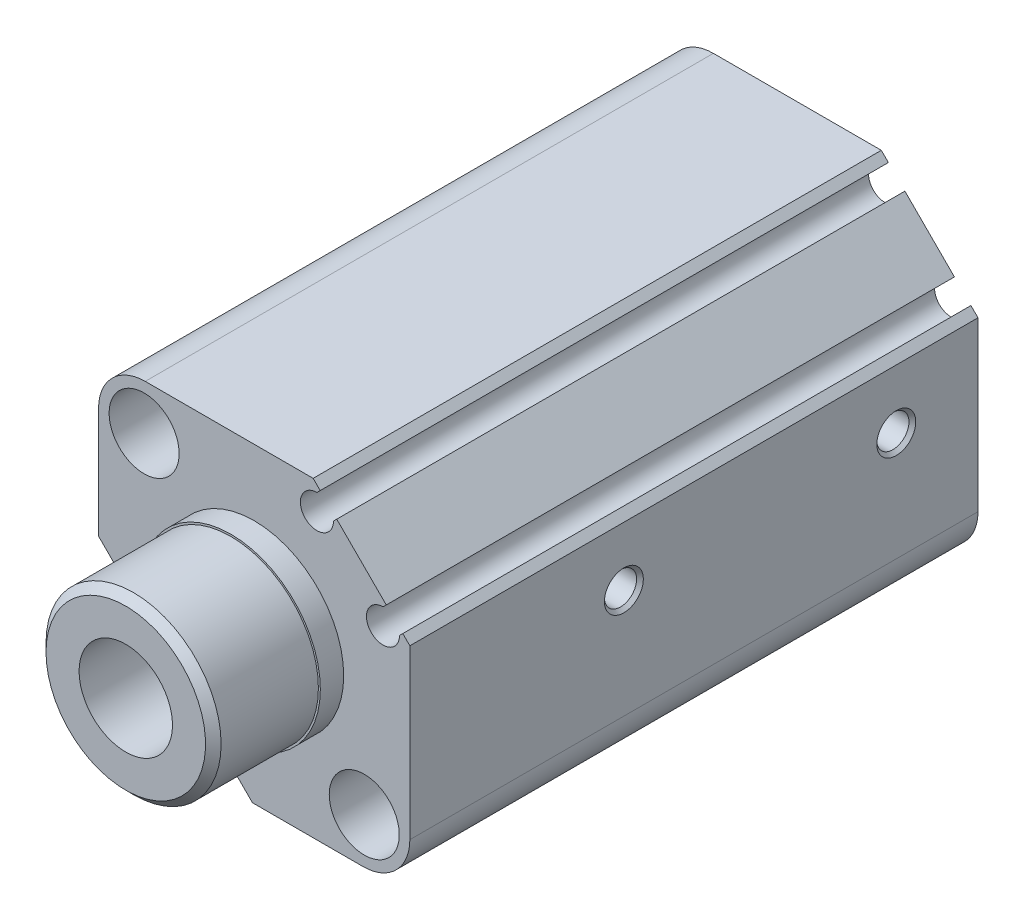
from build123d import *

# Parameters (mm, degrees)
EXTRUDE_1_DEPTH = 73


with BuildPart() as part:
    # 草图1 → 凸台-拉伸1 (new body)
    with BuildSketch(Plane.XY):
        with BuildLine():
            Line((-20, 14), (-20, -0.223253942))
            Line((-20, -0.223253942), (-14.919953083, -5.303300859))
            Line((-14.919953083, -5.303300859), (-19.657568517, -10.040916293))
            Line((-19.657568517, -10.040916293), (-17.960512242, -11.737972568))
            Line((-17.960512242, -11.737972568), (-16.828035921, -10.605496246))
            ThreePointArc((-16.828035921, -10.605496246), (-13.205219139, -9.245421164), (-14.565294221, -12.868237946))
            Line((-14.565294221, -12.868237946), (-15.697770542, -14.000714267))
            Line((-15.697770542, -14.000714267), (-14.000714267, -15.697770542))
            Line((-14.000714267, -15.697770542), (-12.868237946, -14.565294221))
            ThreePointArc((-12.868237946, -14.565294221), (-9.245421164, -13.205219139), (-10.605496246, -16.828035921))
            Line((-10.605496246, -16.828035921), (-11.737972568, -17.960512242))
            Line((-11.737972568, -17.960512242), (-10.040916293, -19.657568517))
            Line((-10.040916293, -19.657568517), (-5.303300859, -14.919953083))
            Line((-5.303300859, -14.919953083), (-0.223253942, -20))
            Line((-0.223253942, -20), (14, -20))
            ThreePointArc((14, -20), (18.242640687, -18.242640687), (20, -14))
            Line((20, -14), (20, 7.577164466))
            Line((20, 7.577164466), (19.091883092, 8.485281374))
            Line((19.091883092, 8.485281374), (18.671295499, 8.064693782))
            ThreePointArc((18.671295499, 8.064693782), (15.04369677, 6.558415396), (16.549975156, 10.186014125))
            Line((16.549975156, 10.186014125), (16.970562748, 10.606601718))
            Line((16.970562748, 10.606601718), (10.606601718, 16.970562748))
            Line((10.606601718, 16.970562748), (10.186014125, 16.549975156))
            ThreePointArc((10.186014125, 16.549975156), (6.558415396, 15.04369677), (8.064693782, 18.671295499))
            Line((8.064693782, 18.671295499), (8.485281374, 19.091883092))
            Line((8.485281374, 19.091883092), (7.577164466, 20))
            Line((7.577164466, 20), (-14, 20))
            ThreePointArc((-14, 20), (-18.242640687, 18.242640687), (-20, 14))
        make_face()
    extrude(amount=-EXTRUDE_1_DEPTH)

    # 草图2 → 切除-旋转1 (revolve, cut)
    with BuildSketch(Plane(origin=(0, 0, 0), x_dir=(0.7071067811865476, -0.7071067811865475, 0), z_dir=(0.7071067811865475, 0.7071067811865476, 0)), mode=Mode.PRIVATE) as cut_revolve_1_sk:
        Polygon((20, 73), (24.5, 73), (24.5, 66), (23, 66), (22.4585, 65.4585), (22.4585, 56), (22.75, 56), (22.75, 17), (22.4585, 17), (22.4585, 7.5415), (23, 7), (24.5, 7), (24.5, 0), (20, 0), align=None)
    revolve(cut_revolve_1_sk.sketch.rotate(Axis((14.142135624, -14.142135624, 0), (0, 0, -1)), 135), axis=Axis((14.142135624, -14.142135624, 0), (0, 0, -1)), mode=Mode.SUBTRACT)

    # 草图3 → 切除-旋转2 (revolve, cut)
    with BuildSketch(Plane(origin=(0, 0, 0), x_dir=(0.7071067811865476, -0.7071067811865475, 0), z_dir=(0.7071067811865475, 0.7071067811865476, 0)), mode=Mode.PRIVATE) as cut_revolve_2_sk:
        Polygon((-20, 73), (-15.5, 73), (-15.5, 66), (-17, 66), (-17.5415, 65.4585), (-17.5415, 56), (-17.25, 56), (-17.25, 17), (-17.5415, 17), (-17.5415, 7.5415), (-17, 7), (-15.5, 7), (-15.5, 0), (-20, 0), align=None)
    revolve(cut_revolve_2_sk.sketch.rotate(Axis((-14.142135624, 14.142135624, 0), (0, 0, -1)), 135), axis=Axis((-14.142135624, 14.142135624, 0), (0, 0, -1)), mode=Mode.SUBTRACT)

    # 草图4 → 旋转1 (revolve)
    with BuildSketch(Plane(origin=(0, 0, 0), x_dir=(1, 0, 0), z_dir=(0, 1, 0)), mode=Mode.PRIVATE) as revolve_1_sk:
        Polygon((0, 0), (11.5, 0), (11.5, -3), (11.25, -3), (11.25, -15.5), (10.25, -16.5), (0, -16.5), align=None)
    revolve(revolve_1_sk.sketch.rotate(Axis((0, 0, 16.5), (0, 0, -1)), 180), axis=Axis((0, 0, 16.5), (0, 0, -1)))

    # 草图5 → 切除-旋转3 (revolve, cut)
    with BuildSketch(Plane(origin=(0, 0, 0), x_dir=(1, 0, 0), z_dir=(0, 1, 0)), mode=Mode.PRIVATE) as cut_revolve_3_sk:
        Polygon((0, 54.5), (12.5, 54.5), (12.5, 20), (6, 20), (6, -16.5), (0, -16.5), align=None)
    revolve(cut_revolve_3_sk.sketch.rotate(Axis((0, 0, 16.5), (0, 0, -1)), 180), axis=Axis((0, 0, 16.5), (0, 0, -1)), mode=Mode.SUBTRACT)

    # 草图6 → 切除-旋转4 (revolve, cut)
    with BuildSketch(Plane(origin=(0, 0, 0), x_dir=(1, 0, 0), z_dir=(0, 1, 0)), mode=Mode.PRIVATE) as cut_revolve_4_sk:
        Polygon((20, 27.5), (20, 25), (19.567, 25.433), (15, 25.433), (13.806616994, 27.5), align=None)
    revolve(cut_revolve_4_sk.sketch.rotate(Axis((13.806616994, 0, -27.5), (1, 0, 0)), 180), axis=Axis((13.806616994, 0, -27.5), (1, 0, 0)), mode=Mode.SUBTRACT)

    # 草图7 → 切除-旋转5 (revolve, cut)
    with BuildSketch(Plane(origin=(0, 0, 0), x_dir=(1, 0, 0), z_dir=(0, 1, 0)), mode=Mode.PRIVATE) as cut_revolve_5_sk:
        Polygon((20, 62.5), (20, 60), (19.567, 60.433), (15, 60.433), (13.806616994, 62.5), align=None)
    revolve(cut_revolve_5_sk.sketch.rotate(Axis((13.806616994, 0, -62.5), (1, 0, 0)), 180), axis=Axis((13.806616994, 0, -62.5), (1, 0, 0)), mode=Mode.SUBTRACT)


solid = part.part
